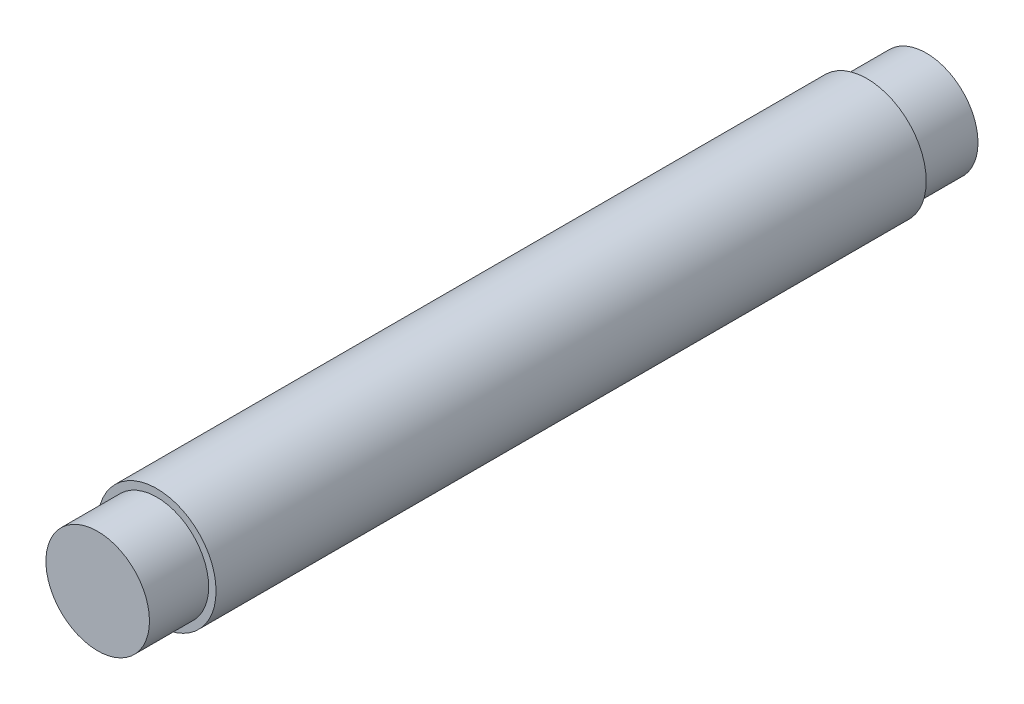
from build123d import *

# Parameters (mm, degrees)
SKETCH1_R           = 87.5
BOSS_EXTRUDE1_DEPTH = 700
SKETCH2_R           = 100
BOSS_EXTRUDE2_DEPTH = 600


with BuildPart() as part:
    # Sketch1 → Boss-Extrude1 (new, symmetric)
    with BuildSketch(Plane.XY):
        Circle(SKETCH1_R)
    extrude(amount=BOSS_EXTRUDE1_DEPTH, both=True)

    # Sketch2 → Boss-Extrude2 (add, symmetric)
    with BuildSketch(Plane.XY):
        Circle(SKETCH2_R)
    extrude(amount=BOSS_EXTRUDE2_DEPTH, both=True)


solid = part.part
